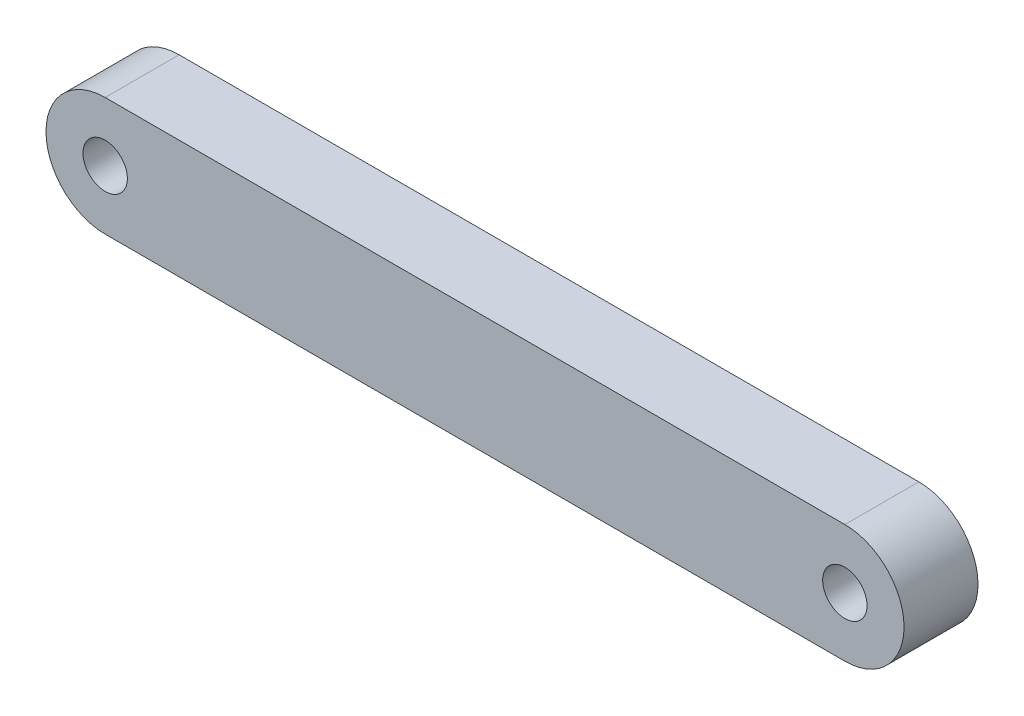
from build123d import *

# Parameters (mm, degrees)
BOSS_EXTRUDE1_DEPTH = 5
SKETCH3_R           = 1.5
CUT_EXTRUDE1_DEPTH  = 30.69848481


with BuildPart() as part:
    # Sketch1 → Boss-Extrude1 (new body)
    with BuildSketch(Plane.XY):
        with BuildLine():
            Line((-25, 4), (25, 4))
            ThreePointArc((25, 4), (29, 0), (25, -4))
            Line((25, -4), (-25, -4))
            ThreePointArc((-25, -4), (-29, 0), (-25, 4))
        make_face()
    extrude(amount=BOSS_EXTRUDE1_DEPTH)

    # Sketch3 → Cut-Extrude1 (cut, through all)
    with BuildSketch(Plane.XY.offset(5)):
        with Locations((-25, 0)):
            Circle(SKETCH3_R)
        with Locations((25, 0)):
            Circle(SKETCH3_R)
    extrude(amount=-CUT_EXTRUDE1_DEPTH, mode=Mode.SUBTRACT)


solid = part.part
